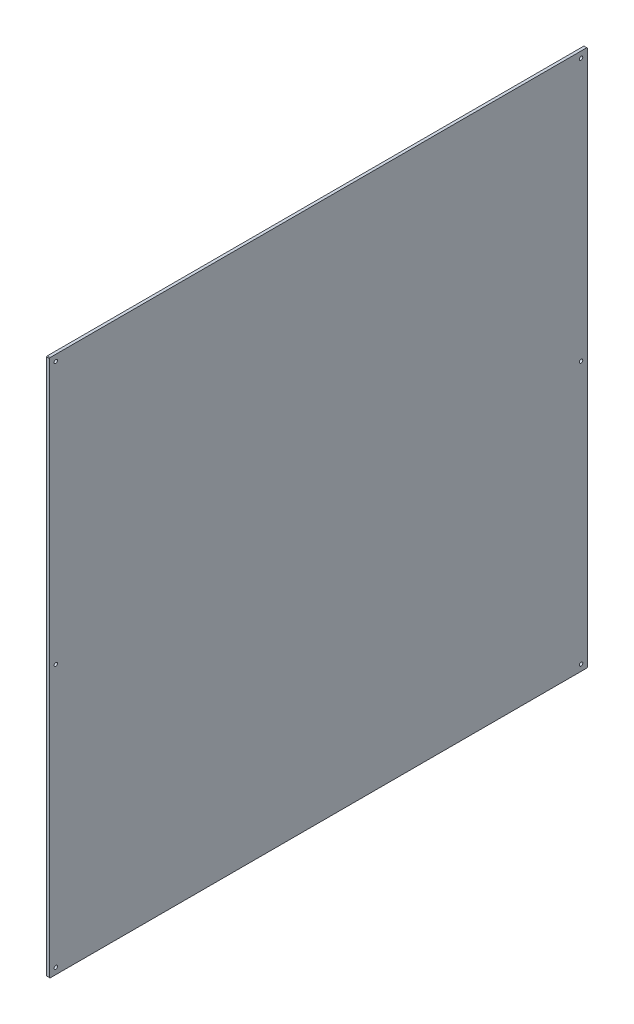
SolidWorks part; units mm, degrees
material "PC(透明)"
ref_plane "前基準面" through (0, 0, 0) normal (0, 0, 1) x (1, 0, 0)
ref_plane "上基準面" through (0, 0, 0) normal (0, 1, 0) x (1, 0, 0)
ref_plane "右基準面" through (0, 0, 0) normal (1, 0, 0) x (0, 0, -1)
sketch "草图1" plane through (0, 0, 0) normal (1, 0, 0) x (0, 0, -1)
  line L1 (469, 468.5) -> (-469, 468.5)
  line L2 (469, 468.5) -> (469, -468.5)
  line L3 (469, -468.5) -> (-469, -468.5)
  line L4 (-469, 468.5) -> (-469, -468.5)
  line L5 (469, 468.5) -> (-469, -468.5) construction
  line L6 (469, -468.5) -> (-469, 468.5) construction
  point P0 (0, 0)
  dimension "D1" = 938
  dimension "D2" = 937
extrude "凸台-拉伸1" add sketch "草图1" along normal blind 5
chamfer "倒角1" distance 1 angle 45 4 edges at (2.5, -468.5, -469) (2.5, -468.5, 469) (2.5, 468.5, -469) (2.5, 468.5, 469)
sketch "草图2" plane through (0, 0, 0) normal (-1, 0, 0) x (0, 0, 1)
  line L0 (-469, -467.5) -> (-469, 467.5) construction
  line L1 (-468, 468.5) -> (468, 468.5) construction
  line L2 (58.8862, 0) -> (0, 0) construction
  line L3 (0, 0) -> (0, 69.8386) construction
  line L5 (458, -457.5) -> (-458, -457.5) construction
  line L6 (458, -457.5) -> (458, 457.5) construction
  line L7 (458, 457.5) -> (-458, 457.5) construction
  line L8 (-458, -457.5) -> (-458, 457.5) construction
  line L9 (458, -457.5) -> (-458, 457.5) construction
  line L10 (458, 457.5) -> (-458, -457.5) construction
  circle A0 centre (-458, 457.5) radius 3
  circle A1 centre (-458, -457.5) radius 3
  circle A2 centre (458, -457.5) radius 3
  circle A3 centre (458, 457.5) radius 3
  circle A8 centre (458, 0) radius 3
  circle A9 centre (-458, 0) radius 3
  dimension "D1" = 6
  dimension "D2" = 11
  dimension "D3" = 11
extrude "切除-拉伸1" cut sketch "草图2" against normal through all
